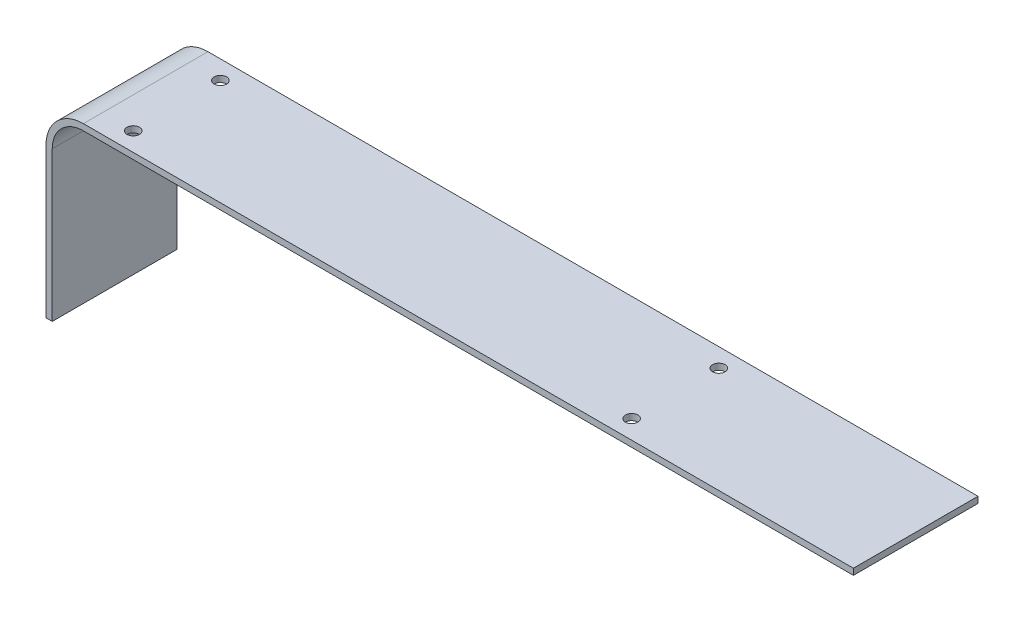
from build123d import *

# Parameters (mm, degrees)
EXTRUDE_THIN1_DEPTH  = 100
SKETCH2_R            = 5
CUT_EXTRUDE1_DEPTH   = 10
LPATTERN1_COUNT      = 2
LPATTERN1_PITCH      = 400
LPATTERN1_COUNT_DIR2 = 2
LPATTERN1_PITCH_DIR2 = 70


with BuildPart() as part:
    # Sketch1 → Extrude-Thin1 (new body)
    with BuildSketch(Plane.XY):
        with BuildLine():
            Line((0, 0), (0, 120))
            ThreePointArc((0, 120), (8.786796564, 141.213203436), (30, 150))
            Line((30, 150), (648, 150))
            Line((648, 150), (648, 145))
            Line((648, 145), (30, 145))
            ThreePointArc((30, 145), (12.32233047, 137.67766953), (5, 120))
            Line((5, 120), (5, 0))
            Line((5, 0), (0, 0))
        make_face()
    extrude(amount=EXTRUDE_THIN1_DEPTH)

    # Sketch2 → Cut-Extrude1 (cut)
    with BuildSketch(Plane.XZ.offset(-145)):
        with Locations(Location((55, 85, 0), (0, 0, 270))):
            Circle(SKETCH2_R)
    cut_extrude1 = extrude(amount=-CUT_EXTRUDE1_DEPTH, mode=Mode.SUBTRACT)

    # LPattern1: Cut-Extrude1 2 × 2
    with Locations(*[(i * LPATTERN1_PITCH, 0, -j * LPATTERN1_PITCH_DIR2) for i in range(LPATTERN1_COUNT) for j in range(LPATTERN1_COUNT_DIR2) if (i, j) != (0, 0)]):
        add(cut_extrude1, mode=Mode.SUBTRACT)


solid = part.part
